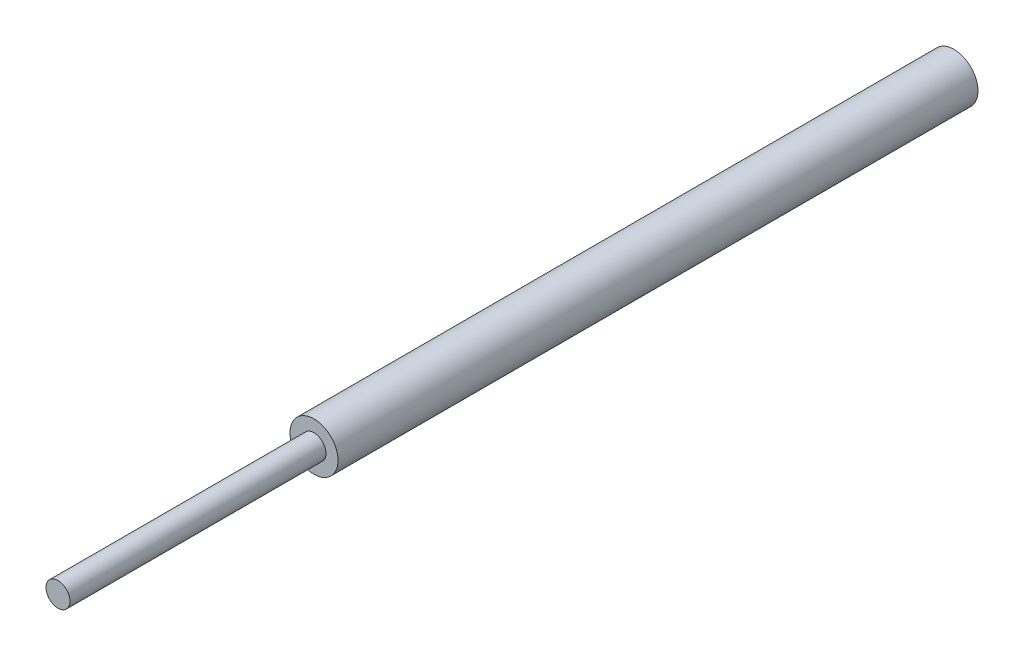
SolidWorks part; units mm, degrees
material "AISI 304"
ref_plane "Front Plane" through (0, 0, 0) normal (0, 0, 1) x (1, 0, 0)
ref_plane "Top Plane" through (0, 0, 0) normal (0, 1, 0) x (1, 0, 0)
ref_plane "Right Plane" through (0, 0, 0) normal (1, 0, 0) x (0, 0, -1)
sketch "Sketch1" plane through (0, 0, 0) normal (0, 0, 1) x (1, 0, 0)
  circle A0 centre (0, 0) radius 1.5
  dimension "D1" = 3
extrude "Boss-Extrude1" add sketch "Sketch1" along normal blind 40
sketch "Sketch2" plane through (0, 0, 40) normal (0, 0, 1) x (1, 0, 0)
  circle A0 centre (0, 0) radius 0.75
  dimension "D1" = 1.5
extrude "Boss-Extrude2" add sketch "Sketch2" along normal blind 16
